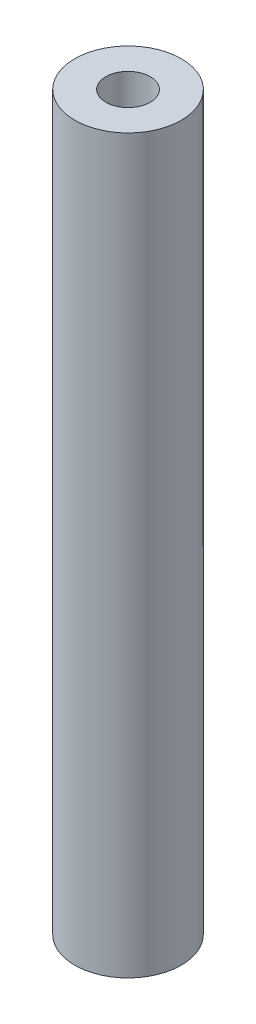
SolidWorks part; units mm, degrees
material "6061 合金"
ref_plane "前视基准面" through (0, 0, 0) normal (0, 0, 1) x (1, 0, 0)
ref_plane "上视基准面" through (0, 0, 0) normal (0, 1, 0) x (1, 0, 0)
ref_plane "右视基准面" through (0, 0, 0) normal (1, 0, 0) x (0, 0, -1)
sketch "草图1" plane through (0, 0, 0) normal (0, 1, 0) x (1, 0, 0)
  circle A0 centre (0, 0) radius 3
  dimension "D1" = 6
extrude "凸台-拉伸1" add sketch "草图1" along normal blind 41.2
sketch "草图2" plane through (0, 41.2, 0) normal (0, 1, 0) x (1, 0, 0)
  point P0 (0, 0)
hole_wizard "M3 螺纹孔1" positions "草图2" profile "草图3" tap size "M3" standard "GB" end condition through all
sketch "草图3" plane through (0, 41.2, 0) normal (1, 0, 0) x (0, 0, 1)
  line L0 (0, 0) -> (0, 41.2)
  line L1 (0, 41.2) -> (1.25, 41.2)
  line L2 (1.25, 41.2) -> (1.25, 0)
  line L5 (1.25, 0) -> (0, 0)
  line L11 (0, -6.35) -> (0, 107.95) construction
  dimension "通孔螺纹孔钻头直径" = 2.5
  dimension "通孔螺纹孔钻头深度" = 41.2
cosmetic thread "孔螺纹线1" parameters "D2"=3
